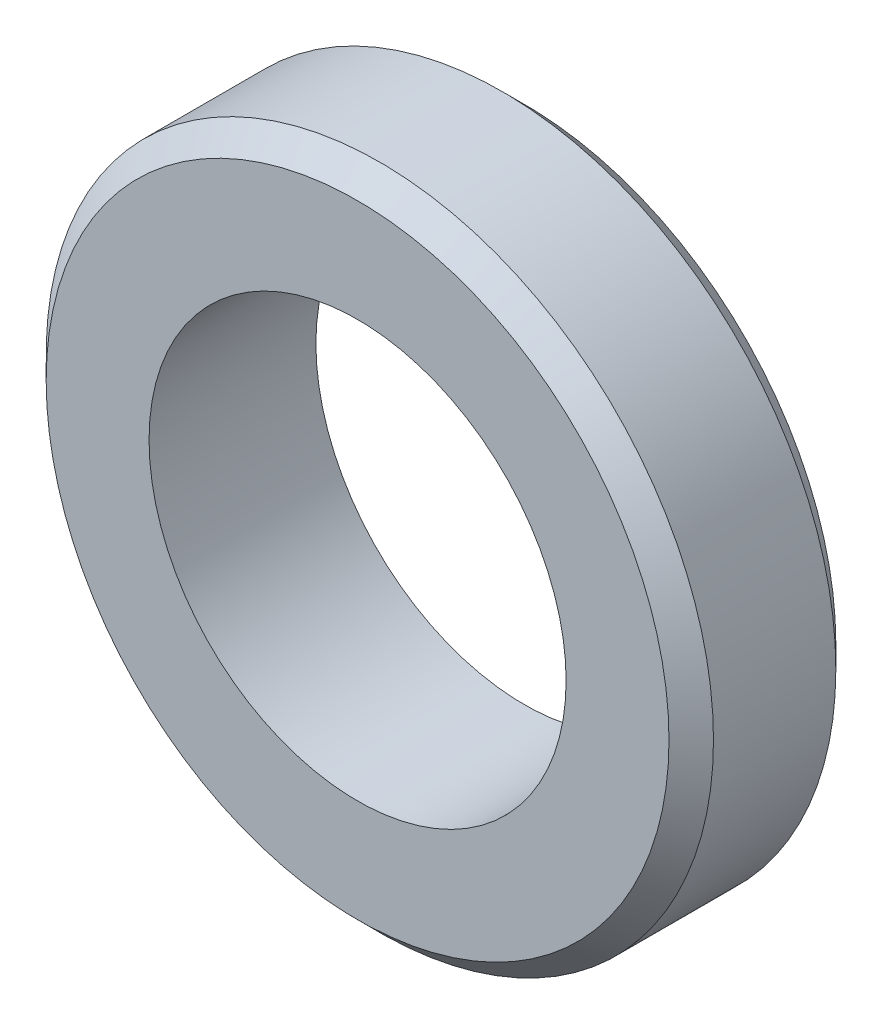
SolidWorks part; units mm, degrees
material "45"
ref_plane "Front Plane" through (0, 0, 0) normal (0, 0, 1) x (1, 0, 0)
ref_plane "Top Plane" through (0, 0, 0) normal (0, 1, 0) x (1, 0, 0)
ref_plane "Right Plane" through (0, 0, 0) normal (1, 0, 0) x (0, 0, -1)
sketch "Sketch1" plane through (0, 0, 0) normal (0, 0, 1) x (1, 0, 0)
  circle A0 centre (0, 0) radius 30
  dimension "D1" = 60
extrude "Boss-Extrude1" add sketch "Sketch1" along normal blind 15
sketch "Sketch2" plane through (0, 0, 15) normal (0, 0, 1) x (1, 0, 0)
  circle A0 centre (0, 0) radius 17.5
  dimension "D1" = 35
extrude "Cut-Extrude1" cut sketch "Sketch2" against normal blind 15
chamfer "Chamfer1" distance 2 angle 45 2 edges at (30, 0, 0) (30, 0, 15)
hole_wizard "M42 Tapped Hole2" positions "Sketch5" profile "Sketch6" tap size "M42" standard "GB"
sketch "Sketch5" plane through (0, 0, 15) normal (0, 0, 1) x (1, 0, 0)
  point P0 (0, 0)
sketch "Sketch6" plane through (0, 0, 15) normal (1, 0, 0) x (0, -1, 0)
  line L0 (0, 0) -> (0, 117.7661)
  line L1 (0, 117.7661) -> (18.75, 106.5)
  line L2 (18.75, 106.5) -> (18.75, 0)
  line L5 (18.75, 0) -> (0, 0)
  line L10 (0, 117.7661) -> (-18.75, 106.5) construction
  line L11 (0, -6.35) -> (0, 107.95) construction
  dimension "螺纹孔钻头直径" = 37.5
  dimension "螺纹孔钻头深度" = 106.5
  dimension "导头角度" = 118
cosmetic thread "Cosmetic thread1" parameters "D1"=15, "D2"=42
